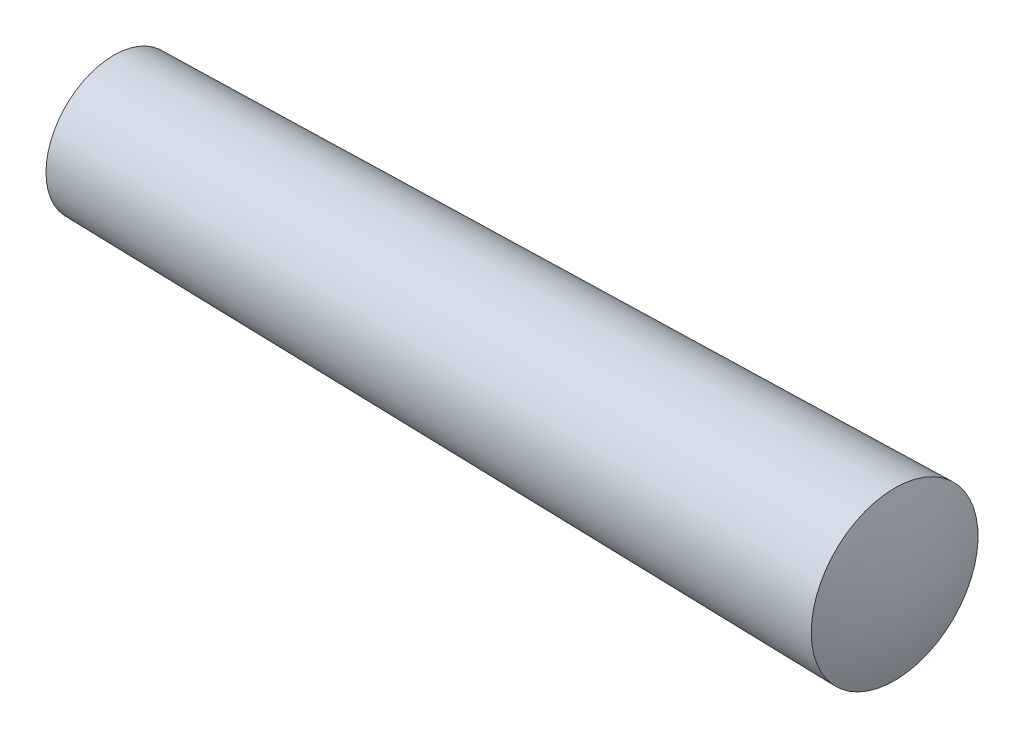
from build123d import *


with BuildPart() as part:
    # Sketch1 → Base-Revolve (revolve)
    with BuildSketch(Plane.XY):
        with BuildLine():
            Line((0, 0), (60, 0))
            ThreePointArc((60, 0), (59.697199442, 3.133971283), (58.8, 6.152))
            Line((58.8, 6.152), (1.2, 5))
            ThreePointArc((1.2, 5), (0.30419989, 2.570992026), (0, 0))
        make_face()
    revolve(axis=Axis((-4.003548939, 0, 0), (1, 0, 0)))


solid = part.part
